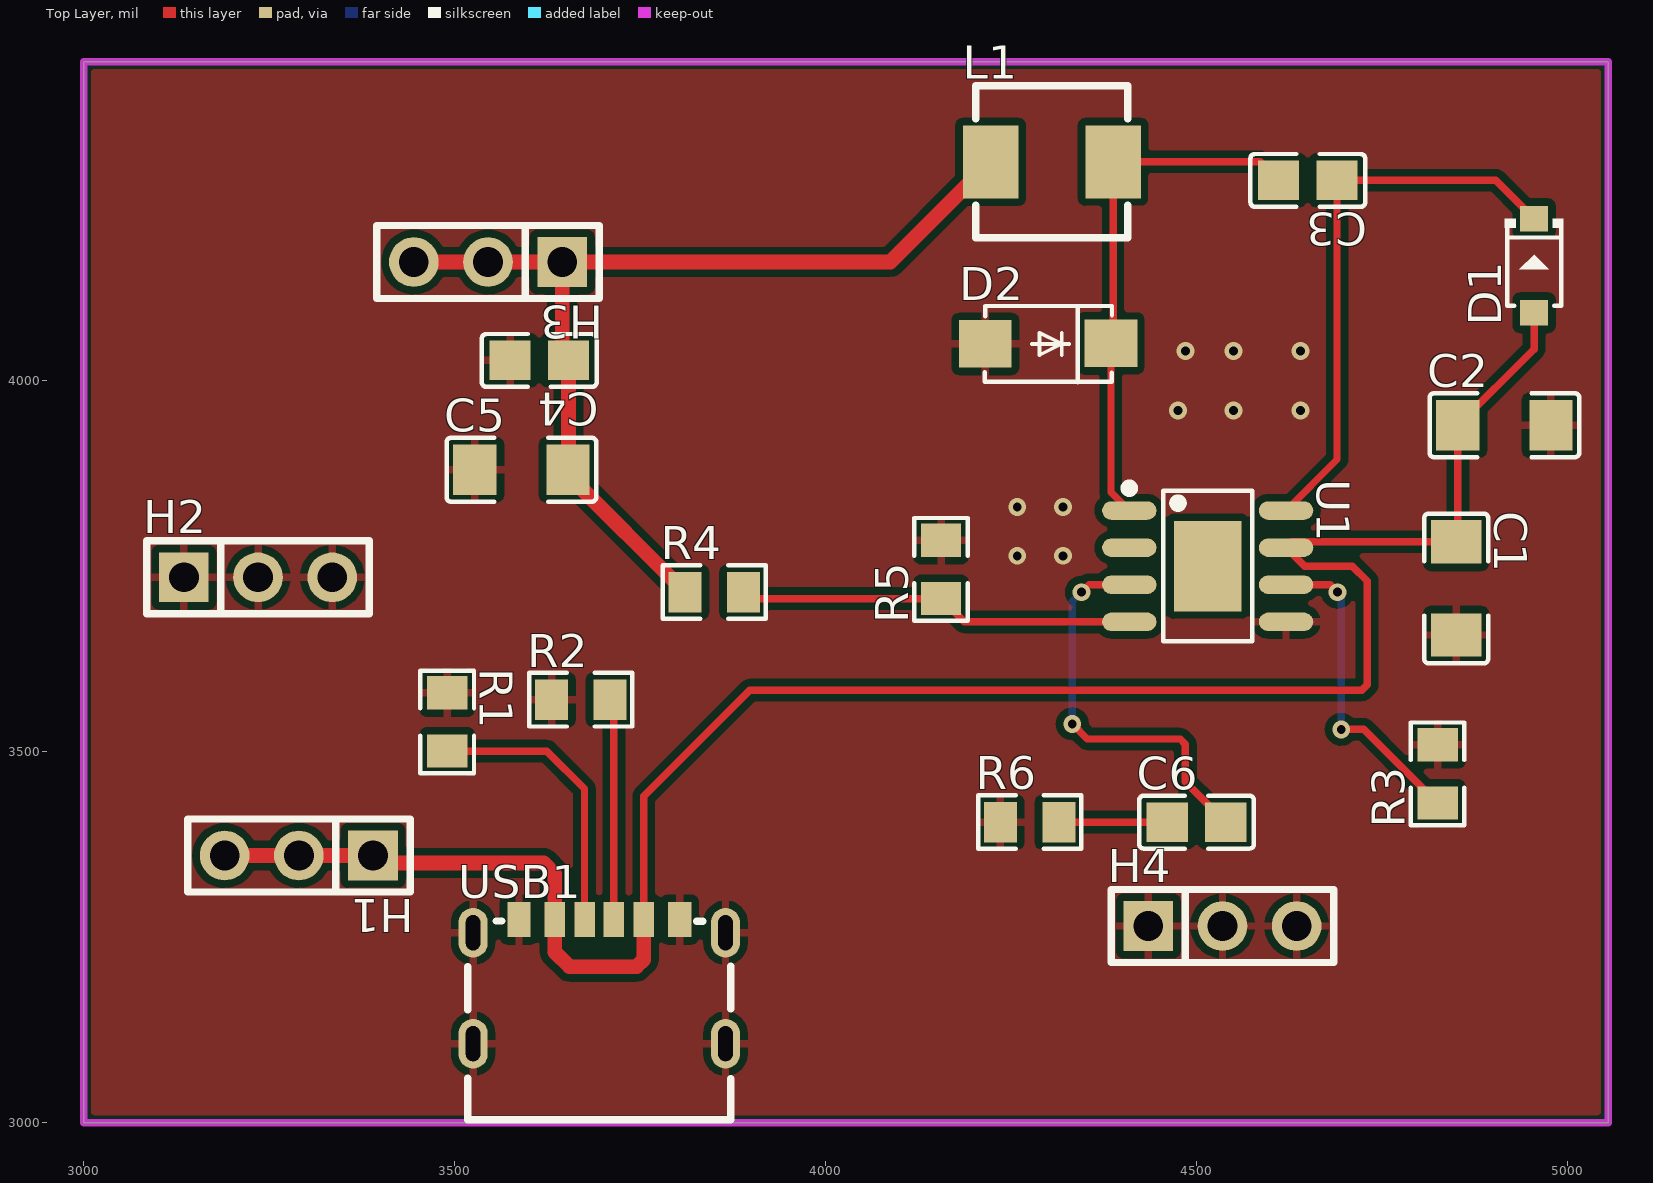
[diagram p0: Top Layer view]
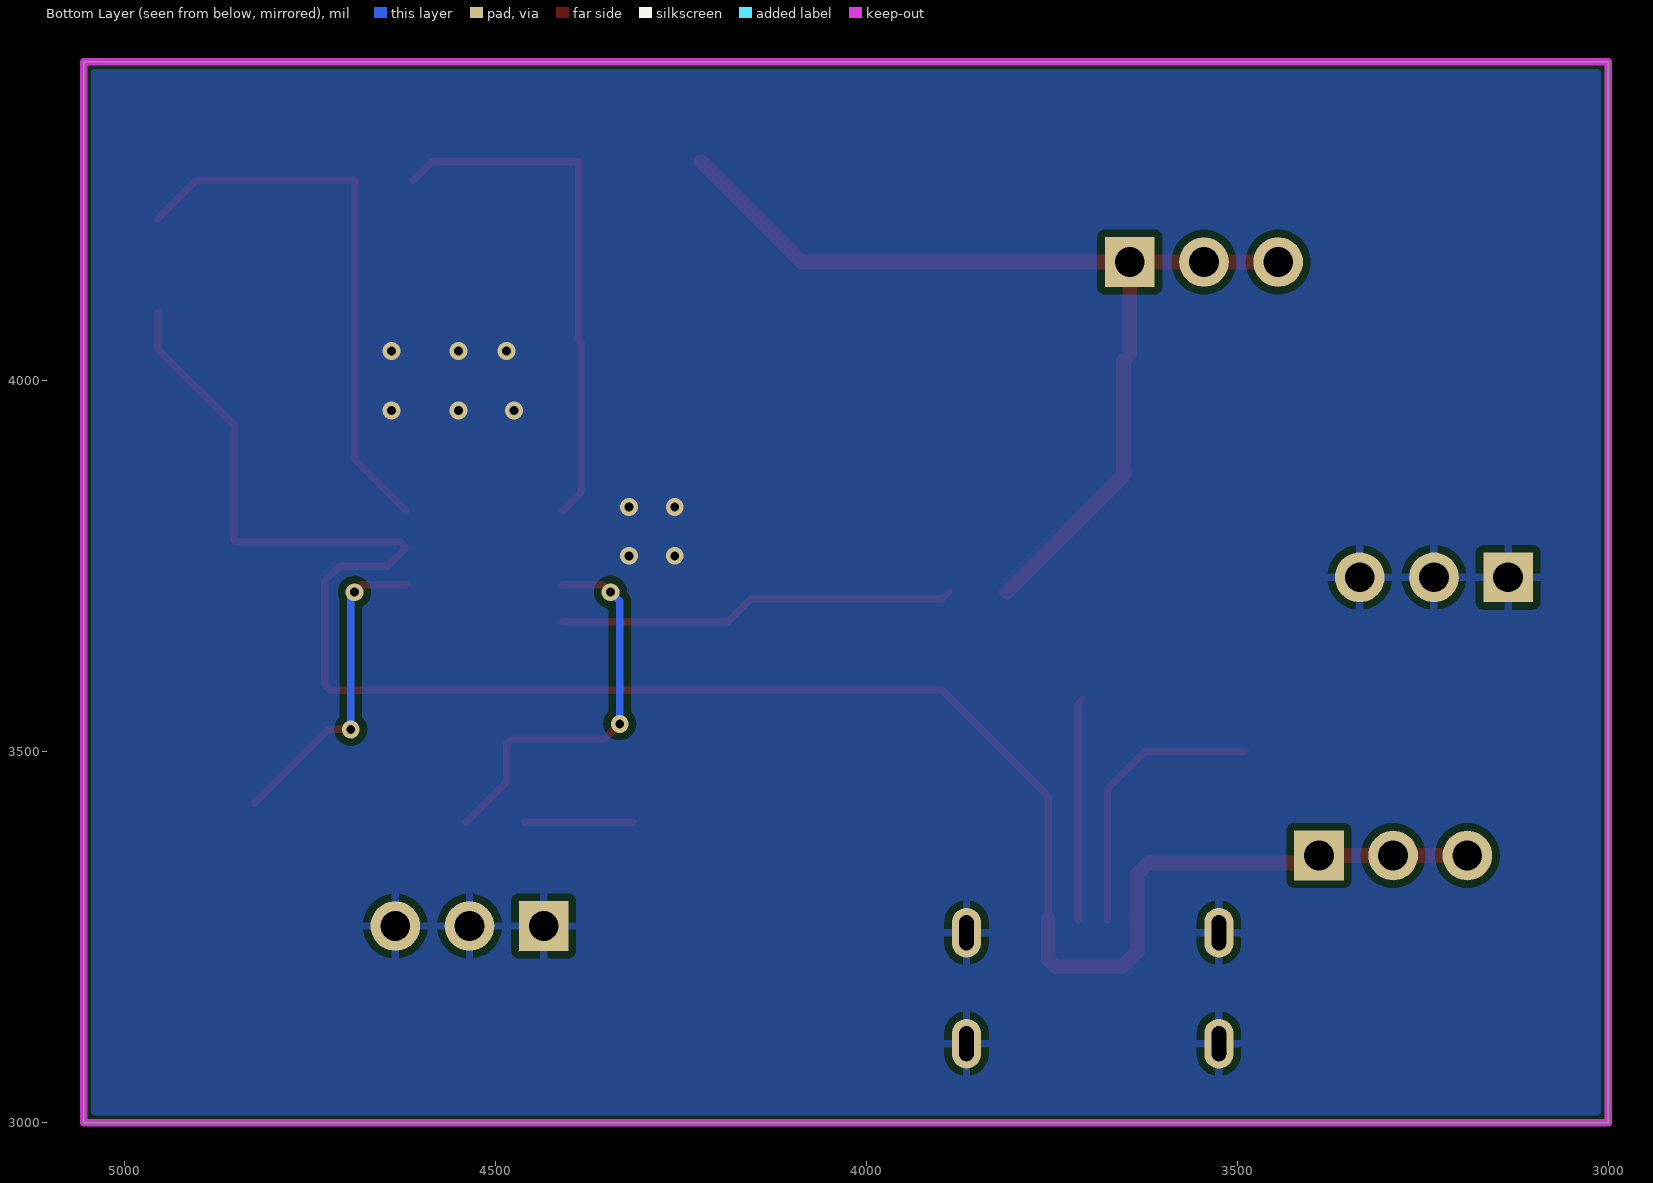
[diagram p1: Bottom Layer view, seen from below]
# Altium PCB MISC51170.pcbdoc
Units mil, origin at the board's own origin, x right, y up, seen from the top; angles counter-clockwise.
Board outline 2055 x 1430 mil, 2 copper layers (Top Layer, Bottom Layer), stack 62.206 mil thick; 21 components, 11 nets, 61 pads, 14 vias.

## Layer stack, top to bottom
Top Solder Mask Layer: solder mask 0.394, Dk 3.3
Top Layer: signal copper 1.379
Dielectric1: surface 59.449, FR4, Dk 4.5
Bottom Layer: signal copper 1.378
Bottom Solder Mask Layer: solder mask 0.394, Dk 3.3

## Board outline
3000,4430 3000,3000 5055,3000 5055,4430

## Design rules (kind name [scope] priority, off if disabled: settings)
BoardOutlineClearance copperThickness2oz_1 [All] p2 off: genericclearance=7.99 ignorepadtopadclearanceinfootprint=FALSE except(0: Arc-SplitContinuation Track-SplitContinuation SMDPad-SplitContinuation THPad-SplitContinuation Via-SplitContinuation Fill-SplitContinuation Region-SplitContinuation Poly-SplitContinuation Text-SplitContinuation Hole-SplitContinuation; 5.98: Arc-CutoutEdge SMDPad-CutoutEdge THPad-CutoutEdge Via-CutoutEdge Fill-CutoutEdge Region-CutoutEdge Text-CutoutEdge; 6.93: Hole-OutlineEdge Hole-CutoutEdge; 10: Poly-OutlineEdge Poly-CutoutEdge; 11.81: Arc-OutlineEdge Track-OutlineEdge SMDPad-OutlineEdge THPad-OutlineEdge Via-OutlineEdge Fill-OutlineEdge Region-OutlineEdge Text-OutlineEdge Track-CutoutEdge)
BoardOutlineClearance copperThickness1oz_1 [All] p4: genericclearance=4.02 ignorepadtopadclearanceinfootprint=FALSE except(0: Arc-SplitContinuation Track-SplitContinuation SMDPad-SplitContinuation THPad-SplitContinuation Via-SplitContinuation Fill-SplitContinuation Region-SplitContinuation Poly-SplitContinuation Text-SplitContinuation Hole-SplitContinuation; 6: SMDPad-CutoutEdge THPad-CutoutEdge Via-CutoutEdge Fill-CutoutEdge Region-CutoutEdge Text-CutoutEdge; 6.93: Hole-OutlineEdge Hole-CutoutEdge; 10: Poly-OutlineEdge Poly-CutoutEdge; 11.8: Arc-OutlineEdge Track-OutlineEdge SMDPad-OutlineEdge THPad-OutlineEdge Via-OutlineEdge Fill-OutlineEdge Region-OutlineEdge Text-OutlineEdge; 11.81: Arc-CutoutEdge Track-CutoutEdge)
Clearance copperThickness2oz [All] p1 off: gap=7.99 ignorepadtopadclearanceinfootprint=FALSE except(5.98: SMDPad-Track SMDPad-SMDPad THPad-Track SMDPad-THPad THPad-THPad Track-Via SMDPad-Via THPad-Via Via-Via Fill-Track Region-Track Fill-SMDPad Region-SMDPad Fill-THPad Region-THPad Fill-Via Region-Via Fill-Fill Fill-Region Region-Region Arc-Track Arc-SMDPad Arc-THPad Arc-Via Fill-Arc Region-Arc Arc-Arc Text-Track SMDPad-Text Text-THPad Text-Via Fill-Text Region-Text Arc-Text Text-Text; 6.93: Hole-Track Hole-SMDPad Hole-THPad Hole-Via Fill-Hole Region-Hole Hole-Arc Hole-Text; 10: Poly-Track Poly-SMDPad Poly-THPad Poly-Via Poly-Fill Poly-Region Poly-Poly Poly-Arc Poly-Text Poly-Hole)
Clearance copperThickness1oz [All] p3: gap=4.02 ignorepadtopadclearanceinfootprint=FALSE except(5.98: SMDPad-Track SMDPad-SMDPad THPad-Track SMDPad-THPad THPad-THPad Track-Via SMDPad-Via THPad-Via Via-Via Fill-Track Region-Track Fill-SMDPad Region-SMDPad Fill-THPad Region-THPad Fill-Via Region-Via Fill-Fill Fill-Region Region-Region; 6: Arc-Track Arc-SMDPad Arc-THPad Arc-Via Fill-Arc Region-Arc Arc-Arc Text-Track SMDPad-Text Text-THPad Text-Via Fill-Text Region-Text Arc-Text Text-Text; 6.93: Hole-Track Hole-SMDPad Hole-THPad Hole-Via Fill-Hole Region-Hole Hole-Arc Hole-Text; 10: Poly-Track Poly-SMDPad Poly-THPad Poly-Via Poly-Fill Poly-Region Poly-Poly Poly-Arc Poly-Text Poly-Hole)
DiffPairsRouting differentialPair [All] p1: maxlimit=6 minlimit=6 mostfreqgap=6 toplayer_minwidth=5 toplayer_prefwidth=10 toplayer_maxwidth=100 toplayer_mingap=6 toplayer_prefgap=6 toplayer_maxgap=6 bottomlayer_minwidth=5 bottomlayer_prefwidth=10 bottomlayer_maxwidth=100 bottomlayer_mingap=6 bottomlayer_prefgap=6 bottomlayer_maxgap=6 maxuncoupledlength=10
HoleToHoleClearance otherClearance [All] p1: gap=11.81 allowstackedmicrovias=TRUE
Length netLength [All] p1: minlimit=0 maxlimit=0
MatchedLengths netLengthTolerance [All] p1: tolerance=1000
PasteMaskExpansion pasteMaskExpansion [All] p1: expansion=0
PlaneConnect innerPlane [All] p1: planeconnectstyle=Relief reliefexpansion=20 reliefentries=4 reliefconductorwidth=10 reliefairgap=10
PolygonConnect copperRegion [(InNet('GND'))] p1: connectstyle=Relief reliefconductorwidth=10 reliefentries=4 polygonreliefangle="90 Angle" airgapwidth=10 via.connectstyle=Relief via.reliefconductorwidth=10 via.reliefentries=4 via.polygonreliefangle="90 Angle" via.airgapwidth=10
RoutingVias viaSize [All] p1: holewidth=12.01 width=24.02 viastyle="Through Hole" minholewidth=11.81 minwidth=19.68 maxholewidth=248.03 maxwidth=393.7
SolderMaskExpansion solderMaskExpansion [IsVia] p1: expansion=-1000 istentingtop=TRUE
SolderMaskExpansion solderMaskExpansion [All] p2: expansion=2 istentingtop=FALSE
Width copperThickness2oz_2 [All] p1 off: maxlimit=100 minlimit=8 preferedwidth=10
Width copperThickness1oz_2 [All] p2: maxlimit=100 minlimit=5 preferedwidth=10

## Components (designator, comment, footprint, x,y, rotation, side; value= is the part's Value field where it differs from the comment)
C1 "4.7uF" C1206 4850,3720 r270 top
C2 "4.7uF" C1206 4915,3940 r0 top
C3 "100nF" C0805 4650,4270 r180 top
C4 "100nF" C0805 3614.04,4027.38 r180 top
C5 "22uF" C1206 3590,3880 r0 top
C6 "680pF" C0805 4500,3405 r0 top
D1 "1N4148W" SOD-123_L2.7-W1.6-LS3.7-FD 4955,4155 r90 top
D2 "SS34" SMA_L4.3-W2.6-LS5.0-FD 4300,4050 r0 top
H1 "PZ254V-11-03P" HDR-TH_3P-P2.54-V-M_PZ254V-11-03P 3290,3360 r180 top
H2 "PZ254V-11-03P" HDR-TH_3P-P2.54-V-M_PZ254V-11-03P 3235,3735 r0 top
H3 "PZ254V-11-03P" HDR-TH_3P-P2.54-V-M_PZ254V-11-03P 3545,4160 r180 top
H4 "PZ254V-11-03P" HDR-TH_3P-P2.54-V-M_PZ254V-11-03P 4535,3265 r0 top
L1 "10uH" IND-SMD_L5.2-W5.2_MCW-0530 4305,4295 r0 top
R1 "5.1kΩ" R0805 3490,3540 r270 top
R2 "5.1kΩ" R0805 3670,3570 r0 top
R3 "200kΩ" R0805 4825,3470 r90 top
R4 "124kΩ" R0805 3850,3715 r0 top
R5 "40.2kΩ" R0805 4155.63,3745.63 r90 top
R6 "42.2kΩ" R0805 4275,3405 r0 top
U1 "MP4560DN-LF-Z" SOIC-8_L4.9-W3.9-P1.27-LS6.0-BL-EP3.1-1 4515,3749.99 r270 top
USB1 "TYPE-C 6P(073)" TYPE-C-SMD_TYPE-C-6P-073 3695,3190 r0 top

## Footprints (in the part's own frame and the unit in brackets; to place one, negate y for a bottom-side part, rotate by r counter-clockwise, add the part's x,y. Pads: shape width x height; smd on the part's side, far side on the other; paste and mask are expansions set on the pad)
C0805 [mm]
  rect 1.41x1.35 smd paste-100 mask+0.051: 1(-1,0) 2(1,0)
  silkscreen extent -1.96,-0.9 1.96,0.9
C1206 [mm]
  rect 1.485x1.728 smd paste-100 mask+0.051: 1(-1.593,0) 2(1.593,0)
  silkscreen extent -2.56,-1.09 2.56,1.09
HDR-TH_3P-P2.54-V-M_PZ254V-11-03P [mm]
  rect 1.7x1.7 hole 1.02: 1(-2.54,0)
  round 1.7 hole 1.02: 2(0,0) 3(2.54,0)
  silkscreen extent -3.81,-1.25 3.81,1.25
IND-SMD_L5.2-W5.2_MCW-0530 [mm]
  rect 1.9x2.5 smd: 1(-2.1,0) 2(2.1,0)
  silkscreen extent -2.6,-2.6 2.6,2.6
R0805 [mm]
  rect 1.133x1.377 smd paste-100 mask+0.051: 1(-1,0) 2(1,0)
  silkscreen extent -1.76,-0.92 1.76,0.92
SMA_L4.3-W2.6-LS5.0-FD [mm]
  rect 1.8x1.62 smd: 1(-2.15,-0.009) 2(2.15,0.009)
  silkscreen extent -2.17,-1.32 2.19,1.29
SOD-123_L2.7-W1.6-LS3.7-FD [mm]
  rect 0.88x0.96 smd: 1(-1.61,0) 2(1.61,0)
  silkscreen extent -1.38,-1 1.6,1
SOIC-8_L4.9-W3.9-P1.27-LS6.0-BL-EP3.1-1 [mm]
  oval 0.63x1.865 smd: 1(-1.905,-2.683) 2(-0.635,-2.683) 3(0.635,-2.683) 4(1.905,-2.683) 5(1.905,2.682) 6(0.635,2.682) 7(-0.635,2.682) 8(-1.905,2.682)
  rect 3.1x2.3 smd paste+0 mask+0.05: 9(0,0)
  silkscreen extent -2.82,-2.83 2.58,1.52
TYPE-C-SMD_TYPE-C-6P-073 [mm]
  oval 1x1.7 hole 0.5 slot 1.2 at 90 deg: 7(-4.32,-2.125) 7(-4.32,1.675) 7(4.32,-2.125) 7(4.32,1.675)
  rect 0.7x1.2 smd paste-100 mask+0.051: A5(-0.5,2.125) A9(1.52,2.125) B5(0.5,2.125) B9(-1.52,2.125)
  rect 0.8x1.2 smd paste-100 mask+0.051: A12(2.75,2.125) B12(-2.75,2.125)
  silkscreen extent -4.5,-4.73 4.5,2.08

## Via types
v1: diameter 24.02, hole 12, Top Layer to Bottom Layer, 14 vias

## Nets (pads, with @x,y where several pads share a name; then routed paths per layer and width w, separated by ;. In a path a pad name is that pad's centre, name@x,y a point inside that pad or via, vN(x,y) a via of type N, cw(c..) or ccw(c..) an arc to the next point about the centre after c; other vN are vias at no path point)
$1N5: R1.2 USB1.A5 | length 382.4
  Top Layer w10: R1.2 3624.37,3500.63 3675,3450 3675,3273.98 USB1.A5
$1N7: R2.2 USB1.B5 | length 298.5
  Top Layer w10: R2.2 3714.68,3564.68 USB1.B5
$1N16: R3.1 U1.6 | length 431.8
  Top Layer w10: U1.6 4680,3725 v1(4690,3715) ; v1(4695,3530) 4725.63,3530 R3.1
  Bottom Layer w10: v1(4690,3715) 4695,3710 v1(4695,3530)
$1N17: C3.1 D1.2 U1.8 | length 760.5
  Top Layer w10: U1.8 4689.37,3893.76 C3.1 4903.39,4270 D1.2
$1N19: C3.2 D2.2 L1.2 U1.1 | length 714.8
  Top Layer w10: U1.1 4384.65,3849.74 D2.2 4387.68,4053.41 L1.2 4585.63,4295 C3.2
$1N24: R4.2 R5.1 U1.4 | length 536.6
  Top Layer w10: R4.2 3898.11,3706.26 R5.1 4186.89,3675 U1.4
$1N33: C6.1 R6.2 | length 146.3
  Top Layer w10: R6.2 C6.1
$1N34: C6.2 U1.3 | length 542.6
  Top Layer w10: v1(4332.5,3537.5) 4352.93,3517.07 4477.93,3517.07 4485,3510 4485,3459.37 C6.2 ; v1(4345,3715) 4355,3725 U1.3
  Bottom Layer w10: v1(4332.5,3537.5) 4332.5,3702.5 v1(4345,3715)
+3.3V: C4.1 C5.2 H3.1 H3.2 H3.3 L1.1 R4.1 | length 1347.4
  Top Layer w20: H3.3 H3.2 H3.1 ; R4.1 3652.7,3872.93 C5.2 3653.41,3880.71 C4.1 3645,4035.79 H3.1 ; L1.1 4087.32,4160 H3.1
GND: C1.2 C2.2 C4.2 C5.1 D2.1 H2.1 H2.2 H2.3 H4.1 H4.2 H4.3 R1.1 R2.1 R3.2 R5.2 R6.1 U1.5 USB1.7 USB1.A12 USB1.B12
  other v1: 4258.28,3763.99 4320.17,3763.99 4258.28,3830 4320,3830 4475,3960 4550,3960 4640,3960 4485,4040 4550,4040 4640,4040
VIN: C1.1 C2.1 D1.1 H1.1 H1.2 H1.3 U1.7 USB1.A9 USB1.B9 | length 2803.1
  Top Layer w10: USB1.A9 3754.84,3439.84 3897.93,3582.93 4722.93,3582.93 4730,3590 4730,3730 4710,3750 4645.6,3750 U1.7 4628.31,3782.7 C1.1 4852.3,3785 C2.1 4955,4042.7 D1.1
  Top Layer w20: H1.3 H1.2 H1.1 3400,3350 3620,3350 3635,3335 3635,3273.82 USB1.B9 3635,3273.51 3635,3230 3655,3210 3745,3210 3754.84,3219.84 USB1.A9
pads on no net: U1.2 U1.9

## Polygon pours and split planes (outlines as drawn)
GND on Top Layer (solid, remove dead copper, pour order 0): 3000,4430 3000,3000 5055,3000 5055,4430
GND on Bottom Layer (solid, remove dead copper, pour order 4): 3000,4430 3000,3000 5055,3000 5055,4430

## Keep-outs
Board Outline Layer:
  the board outline again, w10